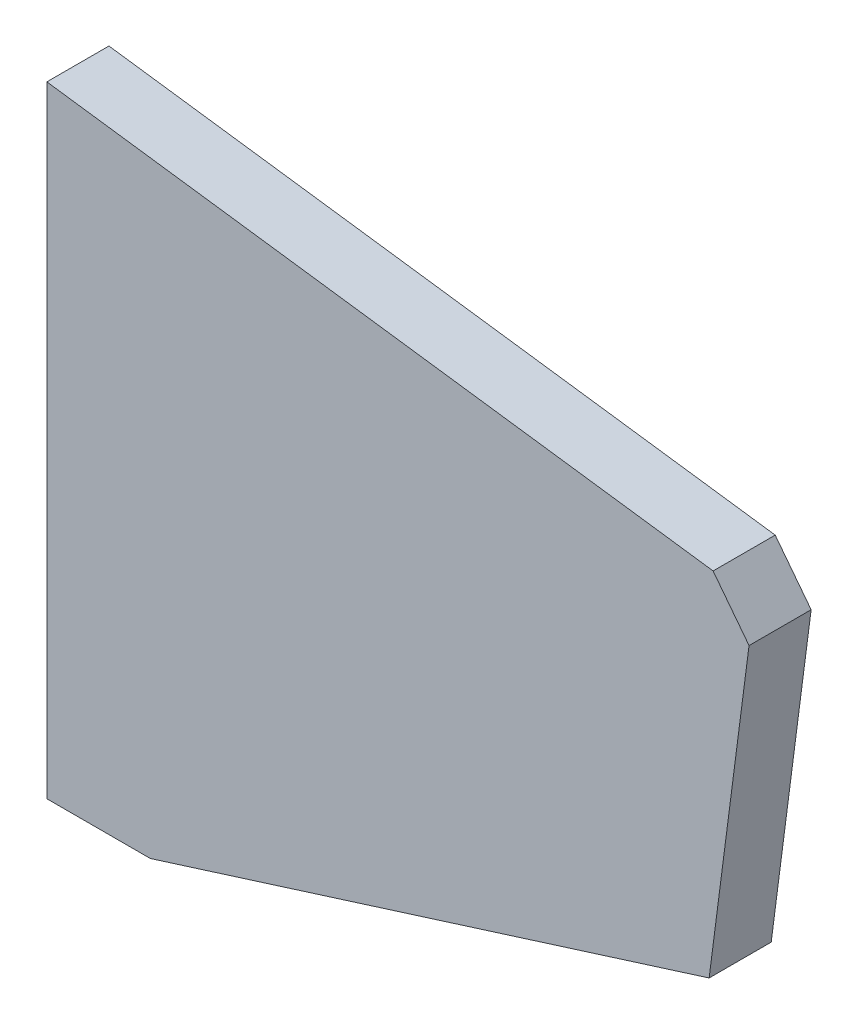
from build123d import *

# Parameters (mm, degrees)
BOSS_EXTRUDE1_DEPTH = 6
CHAMFER1_SIZE       = 4
CHAMFER1_SIZE2      = 4.024049749


with BuildPart() as part:
    # Sketch1 → Boss-Extrude1 (new body)
    with BuildSketch(Plane.XY):
        Polygon((0, 0), (0, 60), (68.372865684, 50.718230869), (64, 17), (10, 0), align=None)
    extrude(amount=BOSS_EXTRUDE1_DEPTH)

    # Chamfer1
    chamfer1_edges = [part.edges().sort_by_distance(p)[0] for p in [
        (68.372865684, 50.718230869, 3),
    ]]
    chamfer1_side = [part.faces().sort_by_distance(p)[0] for p in [
        (66.186432842, 33.859115434, 3),
    ]]
    chamfer(chamfer1_edges, length=CHAMFER1_SIZE, length2=CHAMFER1_SIZE2, reference=chamfer1_side[0])


solid = part.part
